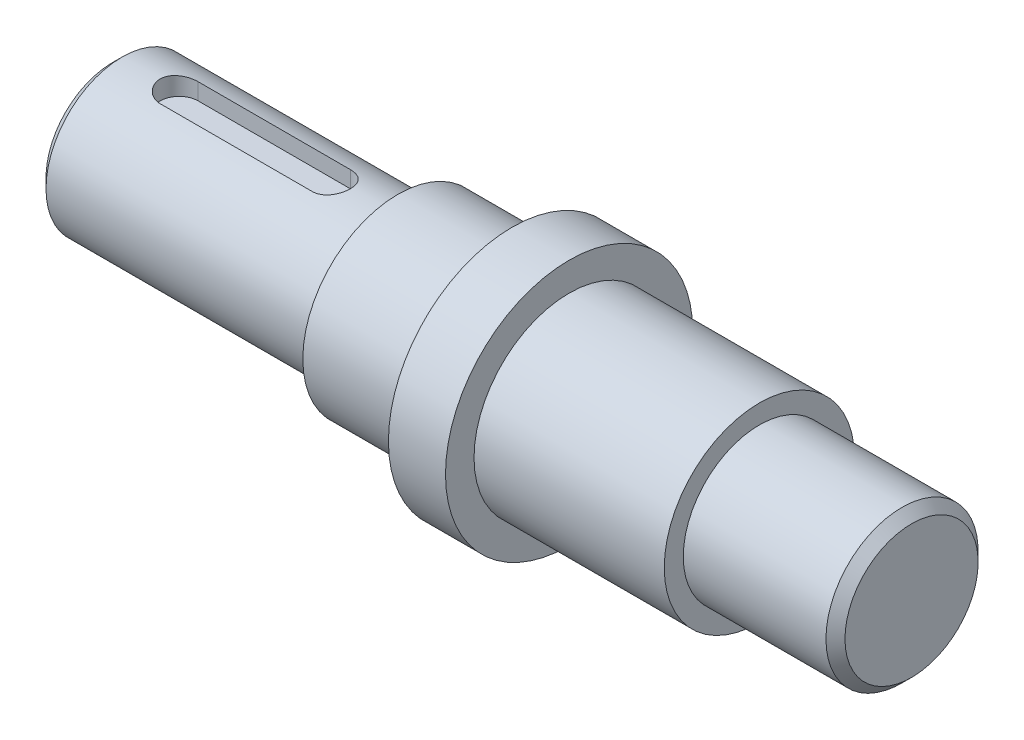
SolidWorks part; units mm, degrees
ref_plane "前视基准面" through (0, 0, 0) normal (0, 0, 1) x (1, 0, 0)
ref_plane "上视基准面" through (0, 0, 0) normal (0, 1, 0) x (1, 0, 0)
ref_plane "右视基准面" through (0, 0, 0) normal (1, 0, 0) x (0, 0, -1)
other "Configuration Table"
sketch "草图1" plane through (0, 0, 0) normal (0, 0, 1) x (1, 0, 0)
  line L0 (-82.0307, 0) -> (84.6321, 0) construction
  line L1 (-23.2676, 0) -> (-23.2676, 4)
  line L2 (-23.2676, 0) -> (18.7324, 0)
  line L3 (-8.2676, 5) -> (-2.2676, 5)
  line L4 (-2.2676, 5) -> (-2.2676, 6.5)
  line L5 (-2.2676, 6.5) -> (0.7324, 6.5)
  line L6 (-8.2676, 4) -> (-8.2676, 5)
  line L7 (0.7324, 6.5) -> (0.7324, 5)
  line L8 (0.7324, 5) -> (10.7324, 5)
  line L9 (10.7324, 4) -> (18.7324, 4)
  line L10 (-23.2676, 4) -> (-8.2676, 4)
  line L11 (18.7324, 4) -> (18.7324, 0)
  line L12 (10.7324, 5) -> (10.7324, 4)
  dimension "D1" = 4
  dimension "D2" = 6
  dimension "D3" = 3
  dimension "D4" = 10
  dimension "D5" = 8
  dimension "D6" = 1
revolve "旋转2" add sketch "草图1" angle 360 about L0
ref_plane "基准面1" through (0, 4, 0) normal (0, 1, 0) x (1, 0, 0)
sketch "草图4" plane through (0, 4, 0) normal (0, 1, 0) x (1, 0, 0)
  line L0 (-23.7327, 0) -> (7.8438, 0) construction
  line L1 (-19.7676, 0) -> (-11.7676, 0) construction
  line L2 (-19.7676, 1) -> (-11.7676, 1)
  line L3 (-19.7676, -1) -> (-11.7676, -1)
  line L4 (-8.2676, 5) -> (-8.2676, -5) construction
  arc A0 (-19.7676, 1) -> (-19.7676, -1) centre (-19.7676, 0) ccw
  arc A1 (-11.7676, -1) -> (-11.7676, 1) centre (-11.7676, 0) ccw
  point P5 (-15.7676, 0)
  dimension "D1" = 3.5
  dimension "D3" = 1
  dimension "D2" = 8
extrude "切除-拉伸3" cut sketch "草图4" against normal blind 1
sketch "草图5" plane through (-23.2676, 0, 0) normal (-1, 0, 0) x (0, 0, 1)
  circle A0 centre (0, 0) radius 1.5
extrude "切除-拉伸4" cut sketch "草图5" against normal blind 10
chamfer "倒角1" distance 0.5 angle 45 1 edges at (-23.2676, 0, 4)
chamfer "倒角2" distance 0.5 angle 45 1 edges at (18.7324, 0, 4)
